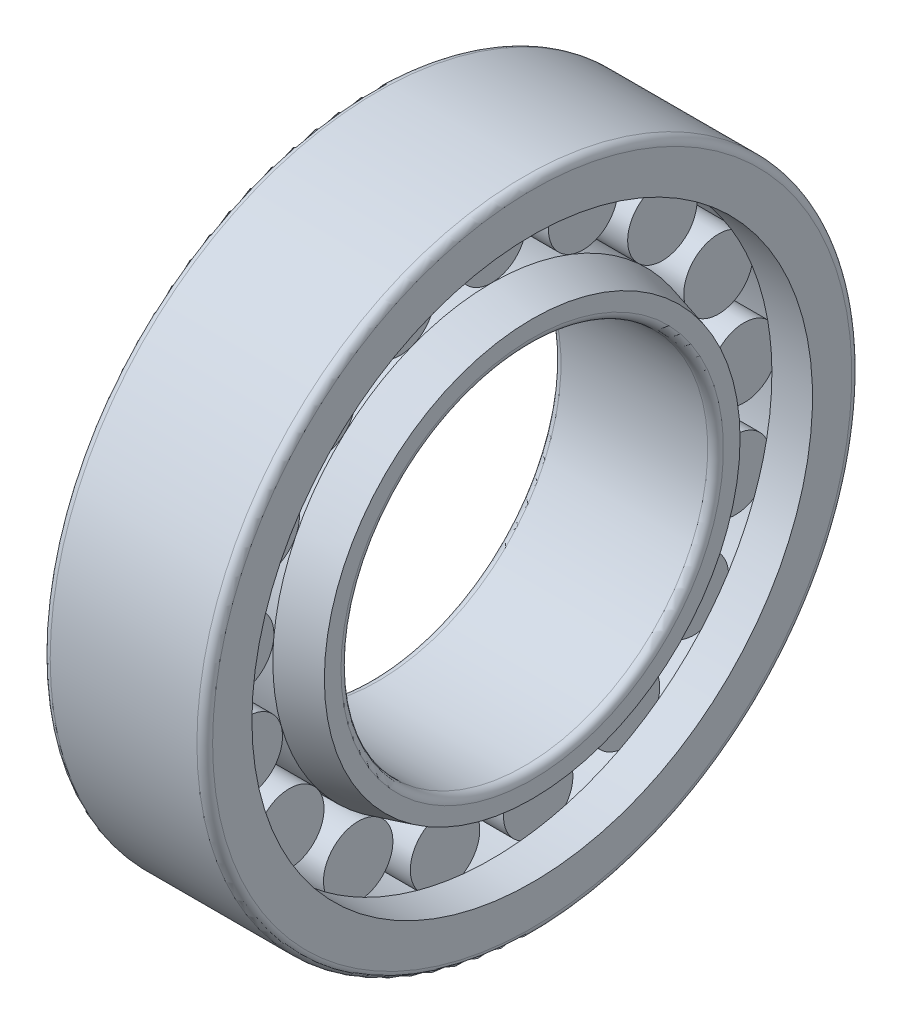
from build123d import *

# Parameters (mm, degrees)
SKETCH3_W         = 15.5
SKETCH3_H         = 6.6251
CIRPATTERN1_COUNT = 17


with BuildPart() as part:
    # Sketch2 → Base-Revolve (revolve)
    with BuildSketch(Plane.XY, mode=Mode.PRIVATE) as base_revolve_sk:
        with BuildLine():
            Line((7.75, 41.75), (23.25, 41.75))
            Line((23.25, 41.75), (31, 39.673393759))
            Line((31, 39.673393759), (31, 36.5))
            ThreePointArc((31, 36.5), (30.560660172, 35.439339828), (29.5, 35))
            Line((29.5, 35), (1.5, 35))
            ThreePointArc((1.5, 35), (0.439339828, 35.439339828), (0, 36.5))
            Line((0, 36.5), (0, 37.383099428))
            Line((0, 37.383099428), (7.75, 41.75))
        make_face()
    revolve(base_revolve_sk.sketch.rotate(Axis((-10.080094127, 0, 0), (1, 0, 0)), 90), axis=Axis((-10.080094127, 0, 0), (1, 0, 0)))

    # Sketch3 → Boss-Revolve1 (revolve)
    with BuildSketch(Plane.XY):
        with Locations((15.5, 45.06245)):
            Rectangle(SKETCH3_W, SKETCH3_H)
    boss_revolve1 = revolve(axis=Axis((-1.603948851, 48.375, 0), (1, 0, 0)))

    # Sketch4 → Boss-Revolve2 (revolve)
    with BuildSketch(Plane.XY, mode=Mode.PRIVATE) as boss_revolve2_sk:
        with BuildLine():
            Line((23.25, 53.5), (31, 53.5))
            Line((31, 53.5), (31, 61))
            ThreePointArc((31, 61), (30.560660172, 62.060660172), (29.5, 62.5))
            Line((29.5, 62.5), (1.5, 62.5))
            ThreePointArc((1.5, 62.5), (0.439339828, 62.060660172), (0, 61))
            Line((0, 61), (0, 53.5))
            Line((0, 53.5), (7.75, 53.5))
            Line((7.75, 53.5), (7.75, 55))
            Line((7.75, 55), (23.25, 55))
            Line((23.25, 55), (23.25, 53.5))
        make_face()
    revolve(boss_revolve2_sk.sketch.rotate(Axis((0, 0, 0), (1, 0, 0)), 90), axis=Axis((0, 0, 0), (1, 0, 0)))

    # CirPattern1: Boss-Revolve1 ×17 about axis
    cirpattern1_axis = Axis((0, 0, 0), (1, 0, 0))
    for i in range(1, CIRPATTERN1_COUNT):
        add(boss_revolve1.rotate(cirpattern1_axis, i * 360 / CIRPATTERN1_COUNT))


solid = part.part
